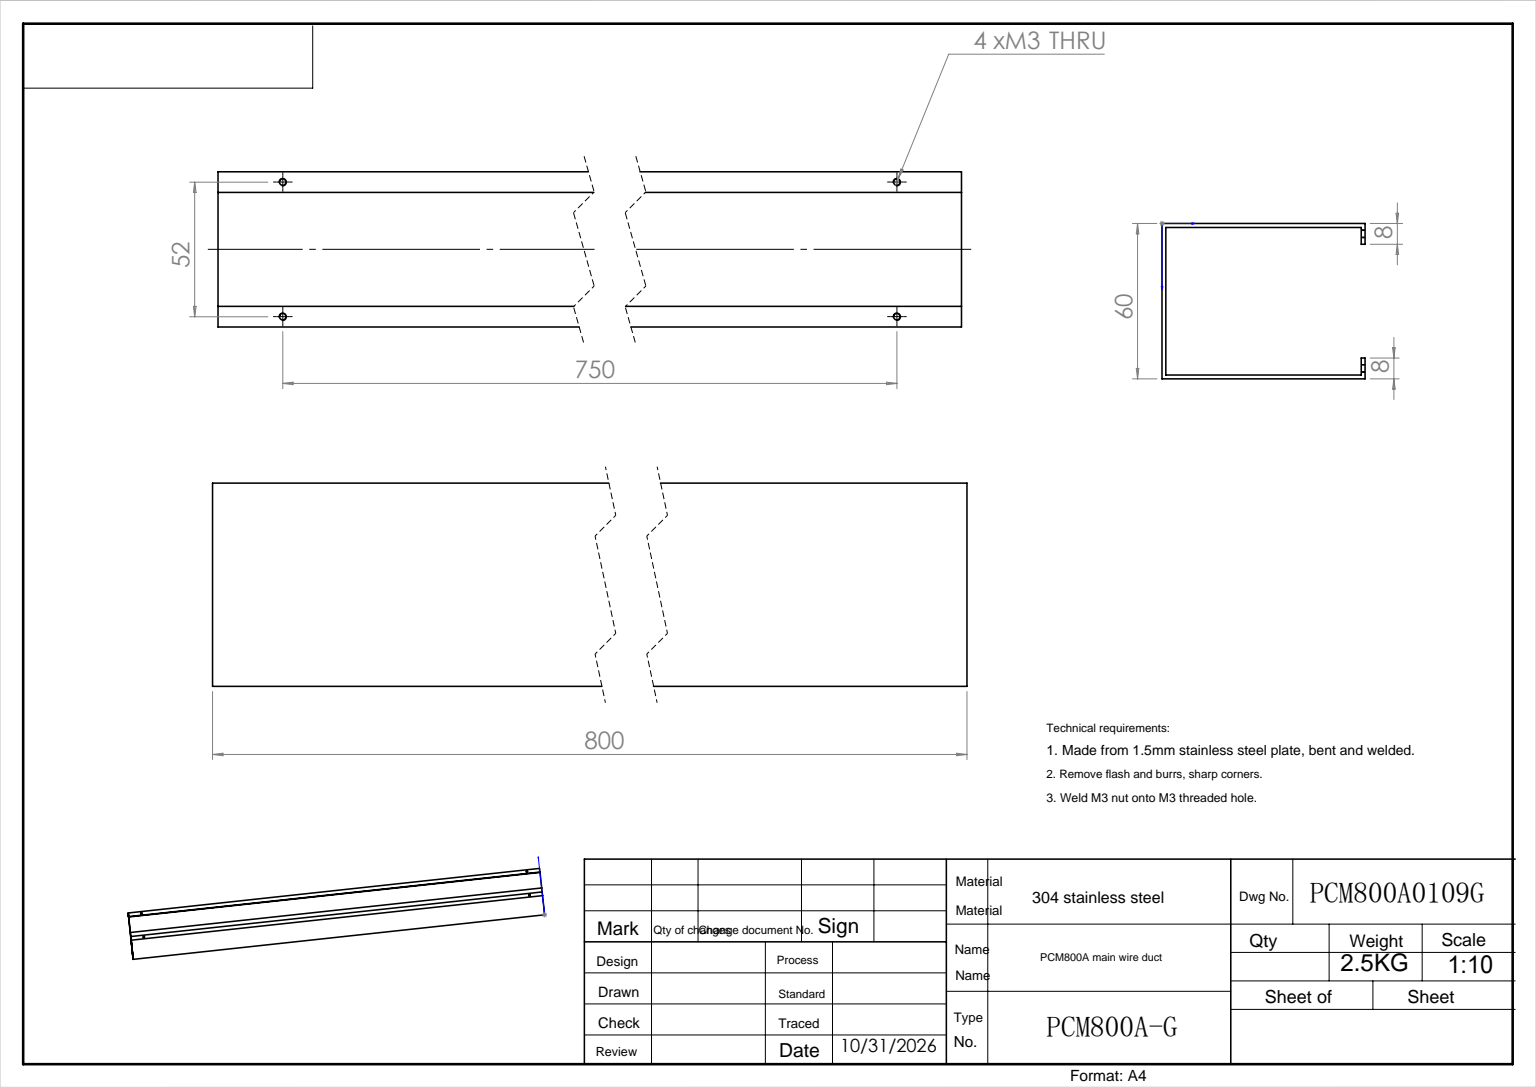
SolidWorks part; units mm, degrees
ref_plane "前视基准面" through (0, 0, 0) normal (0, 0, 1) x (1, 0, 0)
ref_plane "上视基准面" through (0, 0, 0) normal (0, 1, 0) x (1, 0, 0)
ref_plane "右视基准面" through (0, 0, 0) normal (1, 0, 0) x (0, 0, -1)
sketch "草图1" plane through (0, 0, 0) normal (0, 0, 1) x (1, 0, 0)
  line L0 (0, 0) -> (78.5, 0)
  line L1 (78.5, 0) -> (78.5, 8)
  line L2 (0, 0) -> (0, 60)
  line L3 (0, 60) -> (78.5, 60)
  line L4 (78.5, 60) -> (78.5, 52)
  dimension "D1" = 78.5
  dimension "D2" = 60
  dimension "D3" = 78.5
  dimension "D4" = 8
  dimension "D5" = 8
extrude "拉伸-薄壁1" add sketch "草图1" along normal blind 800 thin thin type one direction wall 1.5
hole_wizard "M3 螺纹孔1" positions "草图3" profile "草图2" tap size "M3" standard "GB"
sketch "草图3" plane through (78.5, 0, 0) normal (1, 0, 0) x (0, 0, -1)
  line L0 (0, 60) -> (0, 52) construction
  line L1 (-800, 60) -> (0, 60) construction
  line L2 (-800, 60) -> (-800, 52) construction
  point P0 (-775, 56)
  point P1 (-25, 56)
  dimension "D1" = 4
  dimension "D2" = 25
  dimension "D3" = 4
  dimension "D4" = 25
sketch "草图2" plane through (78.5, 56, 775) normal (0, 1, 0) x (0, 0, -1)
  line L0 (0, 0) -> (0, 78.5)
  line L1 (0, 78.5) -> (1.25, 78.5)
  line L2 (1.25, 78.5) -> (1.25, 0)
  line L5 (1.25, 0) -> (0, 0)
  line L11 (0, -6.35) -> (0, 107.95) construction
  dimension "通孔螺纹孔钻头直径" = 2.5
  dimension "通孔螺纹孔钻头深度" = 78.5
cosmetic thread "孔螺蚊线1" parameters "D2"=3
cosmetic thread "孔螺蚊线2" parameters "D2"=3
ref_plane "基准面2" through (0, 30, 0) normal (0, -1, 0) x (1, 0, 0)
mirror "镜向2" about plane through (0, 30, 0) normal (0, -1, 0) of "M3 螺纹孔1"
